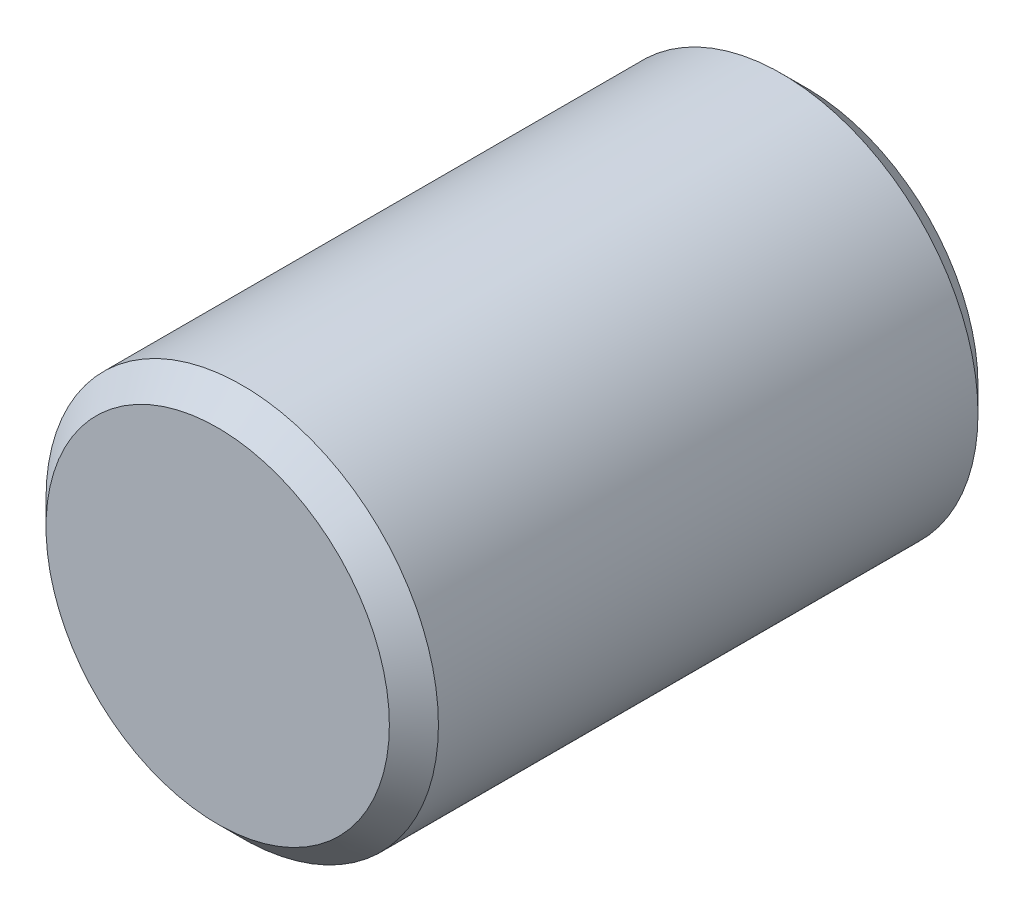
from build123d import *

# Parameters (mm, degrees)
SKETCH1_R           = 4
BOSS_EXTRUDE1_DEPTH = 12
CHAMFER1_SIZE       = 0.5


with BuildPart() as part:
    # Sketch1 → Boss-Extrude1 (new body)
    with BuildSketch(Plane.XY):
        Circle(SKETCH1_R)
    extrude(amount=BOSS_EXTRUDE1_DEPTH)

    # Chamfer1
    chamfer1_edges = [part.edges().sort_by_distance(p)[0] for p in [
        (-4, 0, 0),
        (-4, 0, 12),
    ]]
    chamfer(chamfer1_edges, length=CHAMFER1_SIZE)


solid = part.part
